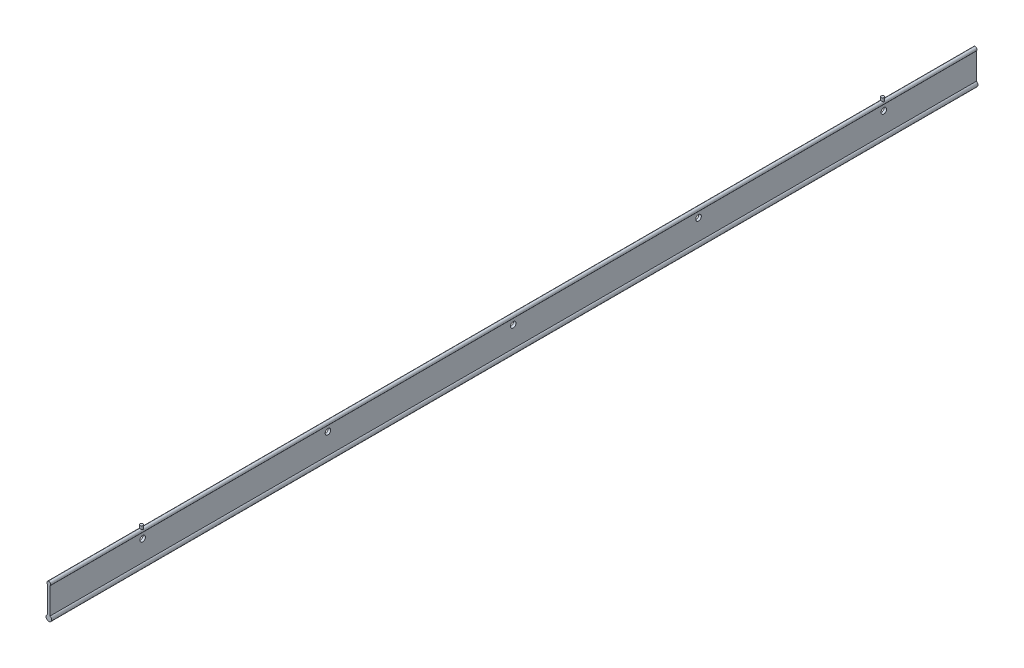
SolidWorks part; units mm, degrees
ref_plane "Front Plane" through (0, 0, 0) normal (0, 0, 1) x (1, 0, 0)
ref_plane "Top Plane" through (0, 0, 0) normal (0, 1, 0) x (1, 0, 0)
ref_plane "Right Plane" through (0, 0, 0) normal (1, 0, 0) x (0, 0, -1)
sketch "Sketch1" plane through (0, 0, 0) normal (0, 0, 1) x (1, 0, 0)
  line L0 (-2.7881, -2.8682) -> (-2.7881, -59.6872)
  line L1 (2.6778, -2.9714) -> (2.6778, -59.6307)
  arc A0 (2.6778, -2.9714) -> (-2.7881, -2.8682) centre (0, 0) ccw
  arc A1 (-2.7881, -59.6872) -> (2.6778, -59.6307) centre (0, -65) ccw
  dimension "D1" = 12
  dimension "D2" = 8
  dimension "D3" = 65
extrude "Boss-Extrude1" add sketch "Sketch1" along normal blind 2000
sketch "Sketch2" plane through (2.6778, 0, 0) normal (1, 0, 0) x (0, 0, -1)
  line L0 (-2000, -2.9714) -> (0, -2.9714) construction
  line L1 (0, -59.6307) -> (0, -2.9714) construction
  circle A0 centre (-200, -14.9714) radius 6
  circle A1 centre (-600, -14.9714) radius 6
  circle A2 centre (-1000, -14.9714) radius 6
  circle A3 centre (-1400, -14.9714) radius 6
  circle A4 centre (-1800, -14.9714) radius 6
  dimension "D1" = 12
  dimension "D2" = 12
  dimension "D3" = 200
  dimension "D4" = 5
extrude "Cut-Extrude1" cut sketch "Sketch2" against normal through all
sketch "Sketch3" plane through (0, 0, 0) normal (0, 1, 0) x (1, 0, 0)
  line L0 (-4, -2000) -> (4, -2000) construction
  line L1 (4, 0) -> (-4, 0) construction
  circle A0 centre (0, -200) radius 3.25
  circle A1 centre (0, -1800) radius 3.25
  dimension "D1" = 6.5
  dimension "D2" = 200
  dimension "D3" = 6.5
  dimension "D4" = 200
extrude "Boss-Extrude2" add sketch "Sketch3" along normal blind 10
